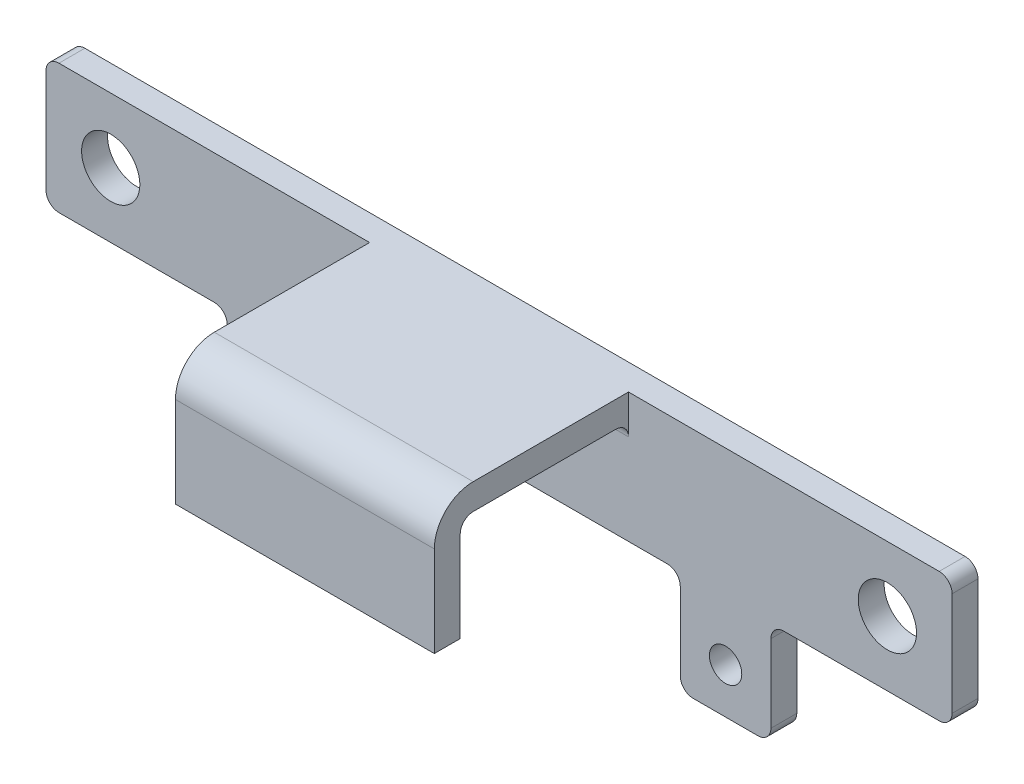
SolidWorks part; units mm, degrees
ref_plane "Front Plane" through (0, 0, 0) normal (0, 0, 1) x (1, 0, 0)
ref_plane "Top Plane" through (0, 0, 0) normal (0, 1, 0) x (1, 0, 0)
ref_plane "Right Plane" through (0, 0, 0) normal (1, 0, 0) x (0, 0, -1)
other "Configuration Table"
sketch "Sketch1" plane through (0, 0, 0) normal (0, 0, 1) x (1, 0, 0)
  line L1 (-35, 5) -> (35, 5)
  line L2 (-35, 5) -> (-35, -5)
  line L3 (-35, -5) -> (35, -5)
  line L4 (35, 5) -> (35, -5)
  line L5 (-35, 5) -> (35, -5) construction
  line L6 (-35, -5) -> (35, 5) construction
  point P0 (0, 0)
  dimension "D1" = 10
  dimension "D2" = 70
extrude "Boss-Extrude1" add sketch "Sketch1" along normal blind 2
sketch "Sketch2" plane through (0, 0, 2) normal (0, 0, 1) x (1, 0, 0)
  line L0 (35, 5) -> (-35, 5) construction
  line L1 (-10, 3) -> (10, 3)
  line L2 (-10, 3) -> (-10, 5)
  line L3 (-10, 5) -> (10, 5)
  line L4 (10, 3) -> (10, 5)
  line L5 (-10, 3) -> (10, 5) construction
  line L6 (-10, 5) -> (10, 3) construction
  point P0 (0, 4)
  dimension "D1" = 2
  dimension "D2" = 20
extrude "Boss-Extrude2" add sketch "Sketch2" along normal blind 15
sketch "Sketch3" plane through (0, 3, 0) normal (0, -1, 0) x (-1, 0, 0)
  line L0 (10, -17) -> (10, -2) construction
  line L1 (10, -15) -> (-10, -15)
  line L2 (10, -15) -> (10, -17)
  line L3 (10, -17) -> (-10, -17)
  line L4 (-10, -15) -> (-10, -17)
  line L5 (10, -15) -> (-10, -17) construction
  line L6 (10, -17) -> (-10, -15) construction
  point P0 (0, -16)
  dimension "D1" = 2
extrude "Boss-Extrude3" add sketch "Sketch3" along normal blind 8
fillet "Fillet2" radius 1 2 edges at (0, 3, 15) (0, 3, 2)
fillet "Fillet3" radius 3 1 edges at (0, 5, 17)
sketch "Sketch4" plane through (0, 0, 2) normal (0, 0, 1) x (1, 0, 0)
  line L0 (35, -5) -> (35, 5) construction
  line L1 (-35, 5) -> (-35, -5) construction
  line L2 (-35, -5) -> (35, -5) construction
  circle A0 centre (-30, 0) radius 2.25
  circle A1 centre (30, 0) radius 2.25
  dimension "D1" = 4.5
  dimension "D2" = 4.5
  dimension "D3" = 5
  dimension "D4" = 5
  dimension "D5" = 5
  dimension "D6" = 5
extrude "Cut-Extrude1" cut sketch "Sketch4" against normal blind 8
sketch "Sketch5" plane through (0, 3, 0) normal (0, -1, 0) x (-1, 0, 0)
  line L0 (35, -2) -> (-35, -2) construction
  line L3 (3.75, -2) -> (-3.75, -2)
sketch "Sketch6" plane through (0, -5, 0) normal (0, -1, 0) x (-1, 0, 0)
  line L0 (35, -2) -> (-35, -2) construction
  line L7 (-21, 0) -> (-14, 0)
  line L8 (-21, 0) -> (-21, -2)
  line L9 (-21, -2) -> (-14, -2)
  line L10 (-14, 0) -> (-14, -2)
  line L11 (-21, 0) -> (-14, -2) construction
  line L12 (-21, -2) -> (-14, 0) construction
  line L14 (14, 0) -> (21, 0)
  line L15 (14, 0) -> (14, -2)
  line L16 (14, -2) -> (21, -2)
  line L17 (21, 0) -> (21, -2)
  line L18 (14, 0) -> (21, -2) construction
  line L19 (14, -2) -> (21, 0) construction
  point P0 (0, -1)
  point P6 (-17.5, -1)
  point P13 (17.5, -1)
  dimension "D1" = 7
  dimension "D2" = 35
  dimension "D3" = 17.5
  dimension "D4" = 7
extrude "Boss-Extrude4" add sketch "Sketch6" along normal blind 8
fillet "Fillet4" radius 1 4 edges at (35, 5, 1) (35, -5, 1) (-35, -5, 1) (-35, 5, 1)
hole_wizard "M3 Tapped Hole1" positions "3DSketch1" profile "Sketch7" tap size "M3" standard "GB"
sketch3d "3DSketch1"
  line L0 (14, -13, 2) -> (14, -5, 2) construction
  line L1 (-21, -13, 2) -> (-21, -5, 2) construction
  point P7 (-17.5, -9.5, 2)
  point P9 (17.5, -9.5, 2)
  dimension "D1" = 3.5
  dimension "D2" = 3.5
sketch "Sketch7" plane through (-17.5, -9.5, 2) normal (1, 0, 0) x (0, -1, 0)
  line L0 (0, 0) -> (0, 8.2511)
  line L1 (0, 8.2511) -> (1.25, 7.5)
  line L2 (1.25, 7.5) -> (1.25, 0)
  line L5 (1.25, 0) -> (0, 0)
  line L10 (0, 8.2511) -> (-1.25, 7.5) construction
  line L11 (0, -6.35) -> (0, 107.95) construction
  dimension "螺纹孔钻头直径" = 2.5
  dimension "螺纹孔钻头深度" = 7.5
  dimension "导头角度" = 118
cosmetic thread "Hole Thread Line 1" parameters "D1"=6, "D2"=3
cosmetic thread "Hole Thread Line 2" parameters "D1"=6, "D2"=3
fillet "Fillet5" radius 1 8 edges at (-21, -5, 1) (-21, -13, 1) (-14, -13, 1) (-14, -5, 1) (14, -5, 1) (21, -5, 1) (14, -13, 1) (21, -13, 1)
